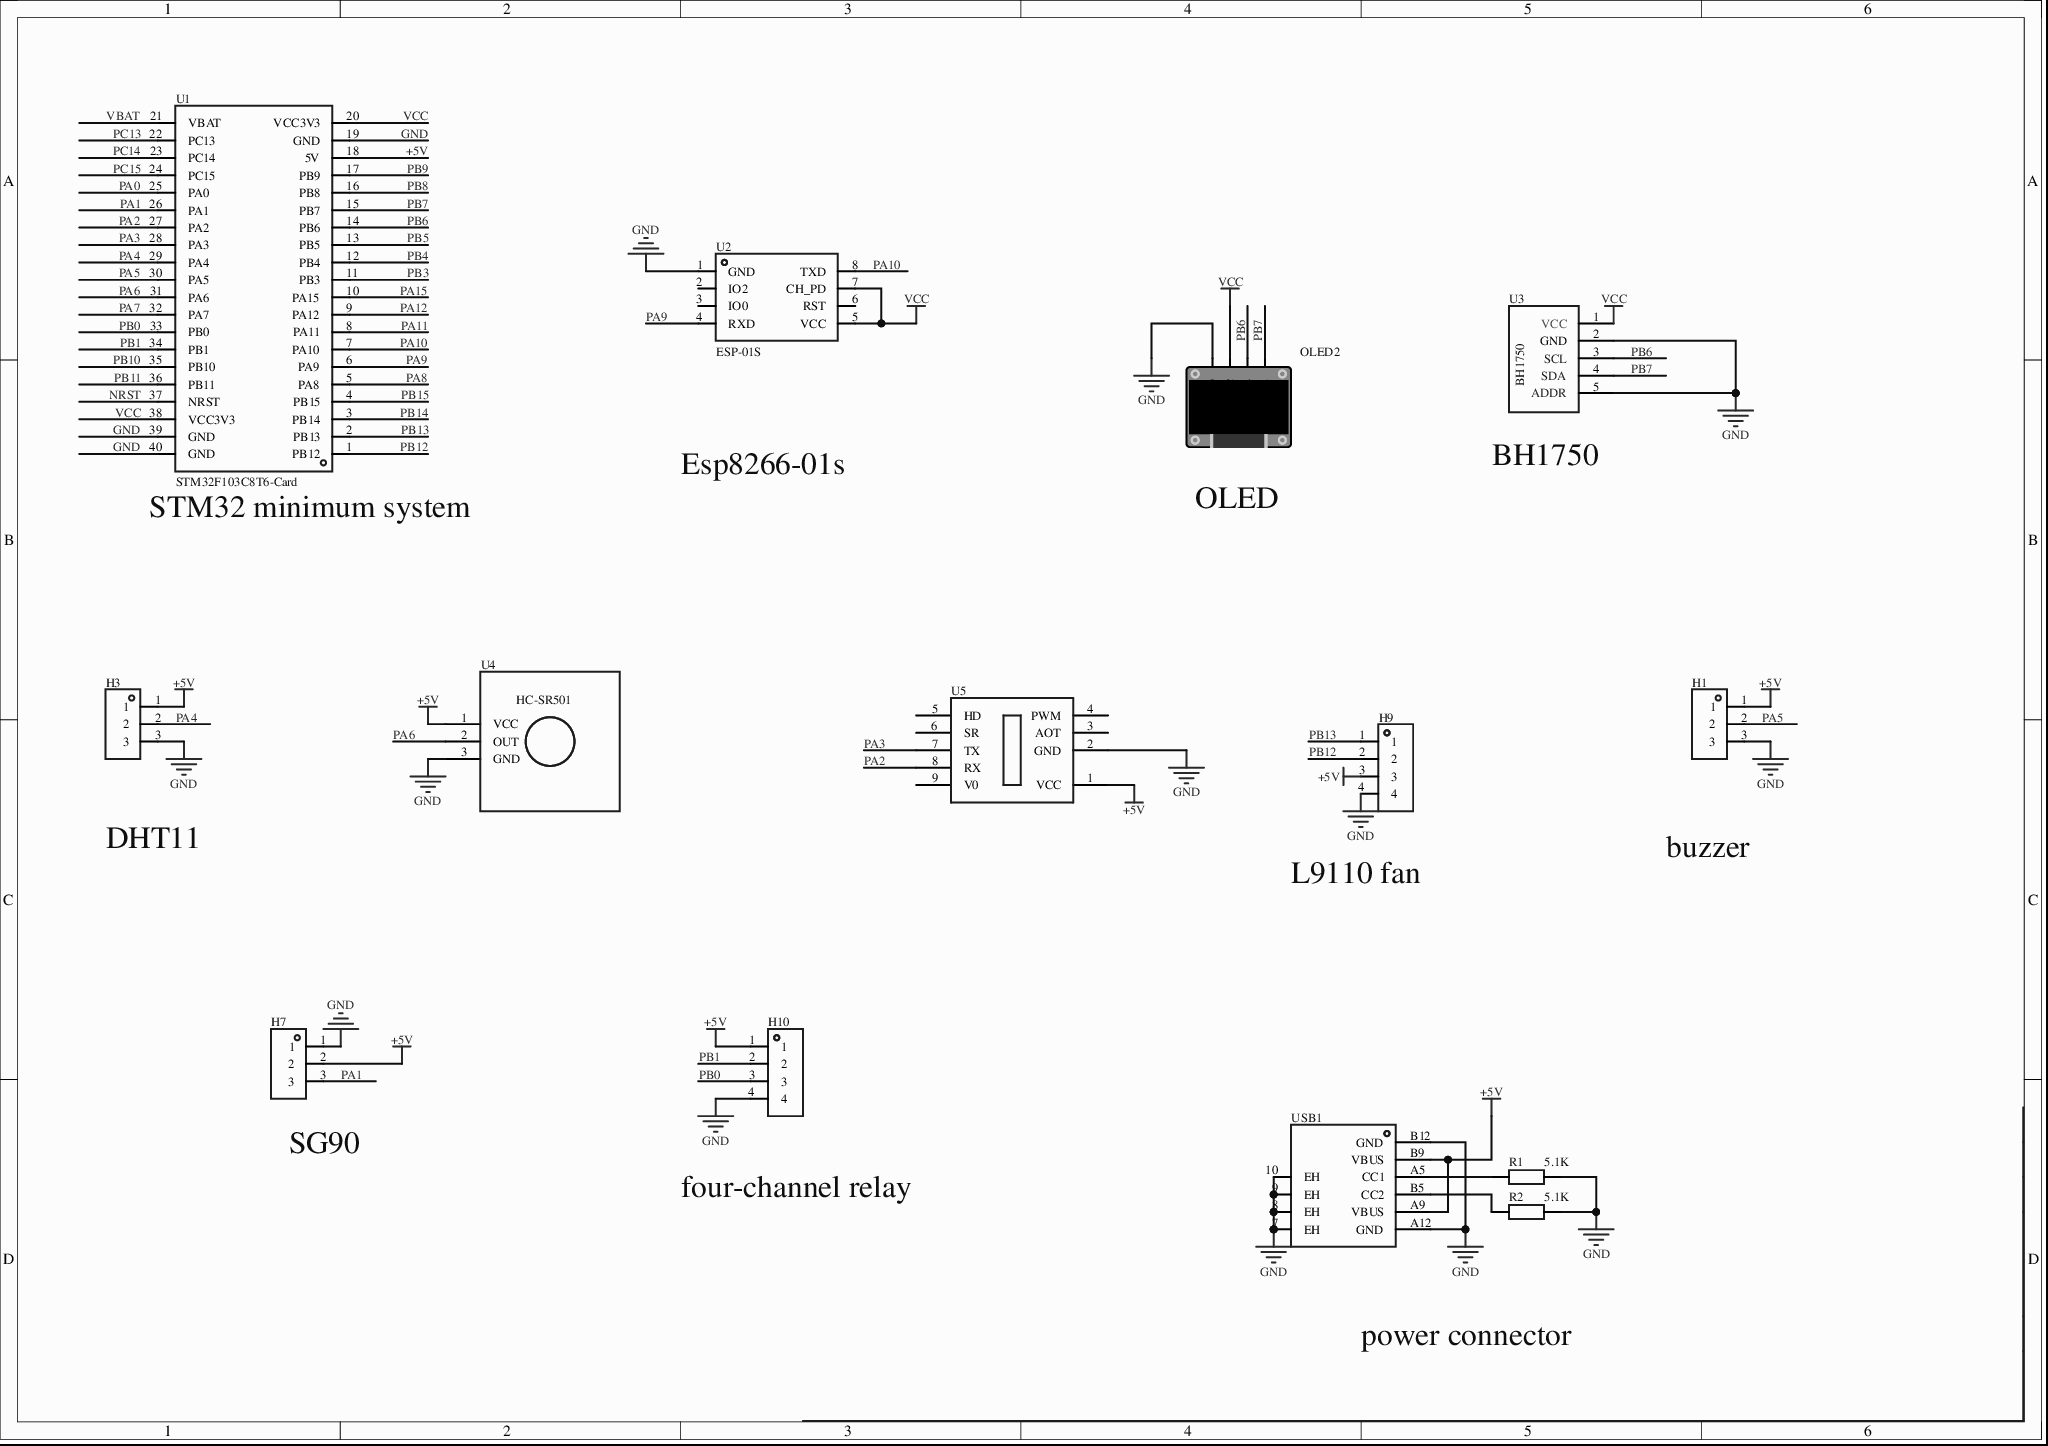
[diagram p0: MISC89045-3.schdoc]
# Altium project MISC89045-2.PrjPcb
1 sheet, 14 parts. Net scope: global (net labels, ports and power ports of the same name join across sheets).
Board file: MISC89045.pcbdoc

## Sheet MISC89045-3.schdoc
size 297 x 209 mm; Version: V1.0; @Project Name: MISC89045; @Page Count: 1; @Update Date: 2026-05-15; @Create Date: 2026-05-15; @Schematic Name: MISC89045; @Page No: 1; @Create Time: 23:22:16; @Update Time: 17:32:40; @Board Name: MISC89045

### Parts
H1  (no value)  [HDR-TH_3P-P2.54-V-F]
H3  (no value)  [HDR-TH_3P-P2.54-V-F]
H7  (no value)  [HDR-TH_3P-P2.54-V-F]
H9  (no value)  [HDR-TH_4P-P2.54-V-F]
H10  (no value)  [HDR-TH_4P-P2.54-V-F]
OLED2  (no value)  [0.96OLED_4P]
R1  5.1K  [R0805]
R2  5.1K  [R0805]
U1  STM32F103C8T6-Card  [CONN-TH_L53.3-W22.9_STM32F103C8T6-CARD]
U2  ESP-01S  [WIFIM-TH_ESP-01S]
U3  (no value)  [BH1750光照传感器]
U4  (no value)  [HC-SR501_W32_H24]
U5  (no value)  [MH-Z19C-9PIN]
USB1  (no value)  [USB_ TYPE-C-6P]

### Nets
+5V: H1.1 H3.1 H7.2 H9.3 H10.1 U1.18(5V) U4.1(VCC) U5.1(VCC) USB1.A9(VBUS) USB1.B9(VBUS)
GND: H1.3 H3.3 H7.1 H9.4 H10.4 OLED2.1(GND) R1.2 R2.2 U1.19(GND) U1.39(GND) U1.40(GND) U2.1(GND) U3.2(GND) U3.5(ADDR) U4.3(GND) U5.2(GND) USB1.7(EH) USB1.8(EH) USB1.9(EH) USB1.10(EH) USB1.A12(GND) USB1.B12(GND)
VCC: OLED2.2(VCC) U1.20(VCC3V3) U1.38(VCC3V3) U2.5(VCC) U2.7(CH_PD) U3.1(VCC)
NRST: U1.37(NRST)
PA0: U1.25(PA0)
PA1: H7.3 U1.26(PA1)
PA2: U1.27(PA2) U5.8(RX)
PA3: U1.28(PA3) U5.7(TX)
PA4: H3.2 U1.29(PA4)
PA5: H1.2 U1.30(PA5)
PA6: U1.31(PA6) U4.2(OUT)
PA7: U1.32(PA7)
PA8: U1.5(PA8)
PA9: U1.6(PA9) U2.4(RXD)
PA10: U1.7(PA10) U2.8(TXD)
PA11: U1.8(PA11)
PA12: U1.9(PA12)
PA15: U1.10(PA15)
PB0: H10.3 U1.33(PB0)
PB1: H10.2 U1.34(PB1)
PB3: U1.11(PB3)
PB4: U1.12(PB4)
PB5: U1.13(PB5)
PB6: OLED2.3(SCL) U1.14(PB6) U3.3(SCL)
PB7: OLED2.4(SDA) U1.15(PB7) U3.4(SDA)
PB8: U1.16(PB8)
PB9: U1.17(PB9)
PB10: U1.35(PB10)
PB11: U1.36(PB11)
PB12: H9.2 U1.1(PB12)
PB13: H9.1 U1.2(PB13)
PB14: U1.3(PB14)
PB15: U1.4(PB15)
PC13: U1.22(PC13)
PC14: U1.23(PC14)
PC15: U1.24(PC15)
VBAT: U1.21(VBAT)
NetR1_1: R1.1 USB1.A5(CC1)
NetR2_1: R2.1 USB1.B5(CC2)

Not connected (* = marked no-connect by the designer): U2 2(IO2)* 3(IO0)* 6(RST)*; U5 3(AOT) 4(PWM) 5(HD) 6(SR) 9(V0)

### Notes on the sheet
- (near U1) STM32 minimum system
- Esp8266-01s
- OLED
- (near U3) BH1750
- DHT11
- buzzer
- (near H9) L9110 fan
- (near H7) SG90
- four-channel relay
- power connector

### Library data of the parts
H1 H3 H7 = HDR-F_2.54_1x3P: Symbol: PM254V-11-03-H85; ConvertToPcb: yes; ModelId: f3b3cc5aae9641bf9e56fc160cef875b; ModelName: HDR2.54-F-LI-1X3P; ModelTransform: 299.9994,100,0,0,0,0,0,0,-118.11; Device: HDR-F_2.54_1x3P; FootprintName: HDR-TH_3P-P2.54-V-F; AddInBom: yes; SupplierPart: C541850; Supplier Footprint: 插件
H9 H10 = HDR-F_2.54_1x4P: Symbol: 2.54-1*4P female; ConvertToPcb: yes; ModelId: d187812051054f85879fcaa51a310d8e0819f05c4eef4c71ace90d822a990e87; ModelTransform: 419.6842,98.464,0,0,0,0,0,0,-118.11; Device: HDR-F_2.54_1x4P; AddInBom: yes; SupplierPart: C2718488; Supplier Footprint: 插件; FootprintName: HDR-TH_4P-P2.54-V-F; ModelName: HDR-TH_4P-P2.54-V-F
OLED2 = 0.96OLED模块_4P: Symbol: 0.96OLED module_4P; ConvertToPcb: yes; ModelId: 79c000fdb68d45a296c2e9bedf4f9055; ModelTransform: 1393.69792,1318.895,0,0,0,0,0,-560.079,-137.795; Device: 0.96OLED module_4P; AddInBom: yes; FootprintName: 0.96OLED_4P; Supplier Footprint: 插件; ModelName: 0.96OLED_4P
R1 R2 = Res_0805: Symbol: resistor; ConvertToPcb: yes; ModelId: 37a81e68749a4138bd2dfa6897b24b85; ModelName: R0805_L2.0-W1.3-H0.6; ModelTransform: 78.74,51.181,0,0,0,0,0,-0.0005,0; Device: Res_0805; Value: 5.1K; AddInBom: yes; Supplier Footprint: 0805; FootprintName: R0805
U1 = STM32F103C8T6-Card: AddInBom: yes; Device: STM32F103C8T6-Card; Symbol: STM32F103C8T6-CARD; FootprintName: CONN-TH_L53.3-W22.9_STM32F103C8T6-CARD; LCSC Part Name: STM32F103C8T6-Card; SupplierPart: C9900077949; ManufacturerPart: STM32F103C8T6-Card; Supplier Footprint: 插件; Supplier: LCSC; ConvertToPcb: yes
U2 = ESP-01S_C111009: AddInBom: yes; ModelId: eb7175da78ae48b3b1568cfe3027405f0819f05c4eef4c71ace90d822a990e87; ModelTransform: 582.676,976.37608,0,0,0,0,0,388.346,-118.11; Symbol: ESP-01S; Device: ESP-01S_C111009; LCSC Part Name: ESP-01S; SupplierPart: C111009; ManufacturerPart: ESP-01S; Supplier Footprint: -; JLCPCB Part Class: Extended Part; Supplier: LCSC; ConvertToPcb: yes; FootprintName: WIFIM-TH_ESP-01S; ModelName: WIFIM-TH_ESP-01S
U3 = BH1750光照传感器: Symbol: BH1750 light sensor; AddInBom: yes; Device: BH1750 light sensor; ConvertToPcb: yes; FootprintName: BH1750 light sensor
U4 = HC-SR501: AddInBom: yes; ModelId: bd3632e38f3746bf9e8ddb03d9da7ac386d42a7c85f04678a27c71665693640c; ModelTransform: 1287.39901,980.3129697240615,956.6909550732486,0,90,0,35.43307,881.88976,444.88189; Symbol: HC-SR501; Device: HC-SR501; ConvertToPcb: yes; ModelName: hc-sr501; FootprintName: HC-SR501_W32_H24
U5 = MH-Z19C: Symbol: MH-Z19C; Device: MH-Z19C; FootprintName: MH-Z19C-9PIN
USB1 = USB_ Type-C-6P: AddInBom: yes; ModelId: d4f492a4e6024845a13b3f6a4ef2d2cb0819f05c4eef4c71ace90d822a990e87; ModelName: USB-SMD_U262-061N-4BVC11; ModelTransform: 352.362,281.496,0,0,0,0,0,-47.244,-39.37; Symbol: USB_ TYPE-C-6P; Device: USB_ Type-C-6P; Supplier Footprint: SMD; ConvertToPcb: yes; FootprintName: USB_ TYPE-C-6P